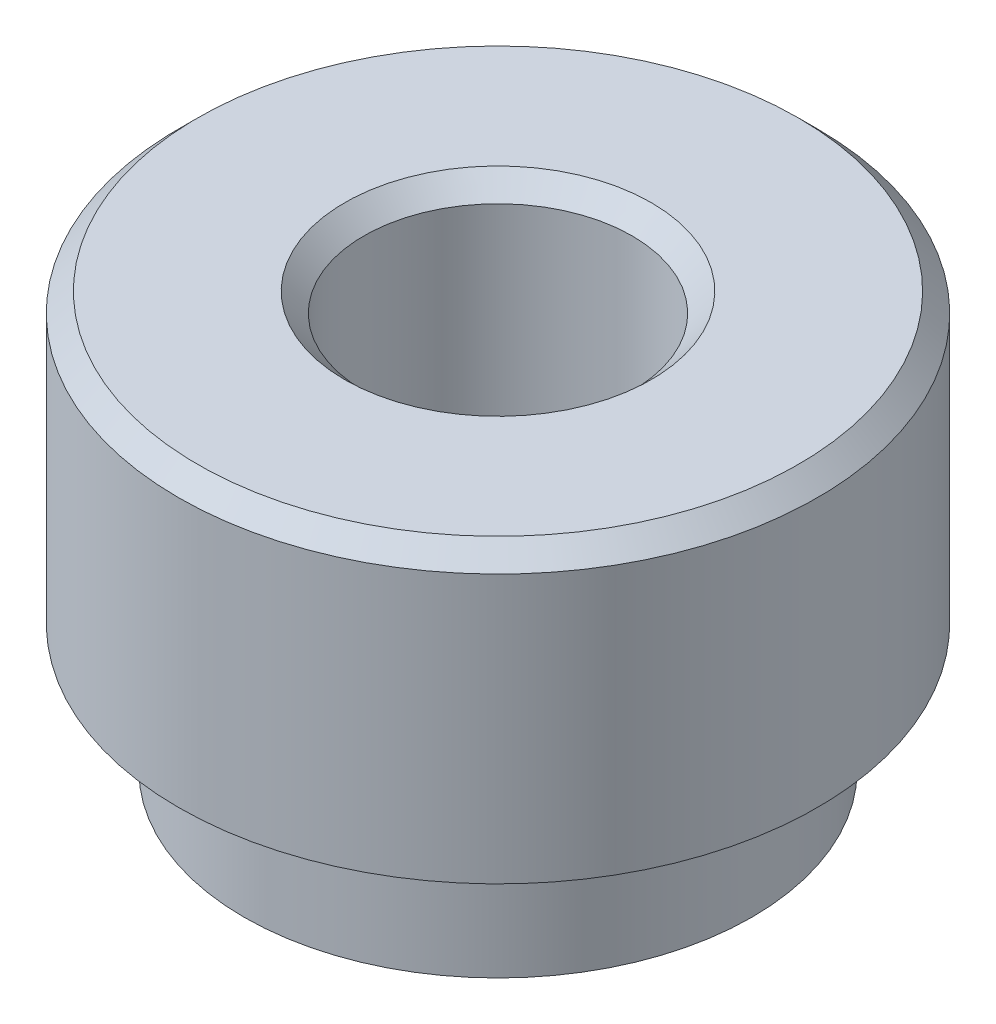
SolidWorks part; units mm, degrees
ref_plane "前视基准面" through (0, 0, 0) normal (0, 0, 1) x (1, 0, 0)
ref_plane "上视基准面" through (0, 0, 0) normal (0, 1, 0) x (1, 0, 0)
ref_plane "右视基准面" through (0, 0, 0) normal (1, 0, 0) x (0, 0, -1)
sketch "草图1" plane through (0, 0, 0) normal (0, 0, 1) x (1, 0, 0)
  line L0 (0, 0) -> (0, 56.263) construction
  line L1 (0, 6.5) -> (-5, 6.5)
  line L2 (-5, 6.5) -> (-5, 2)
  line L3 (-5, 2) -> (-3.975, 2)
  line L4 (-3.975, 2) -> (-3.975, 0)
  line L5 (-3.975, 0) -> (-3.25, 0)
  line L6 (0, 6.5) -> (0, 2)
  line L7 (-3.25, 0) -> (-3.25, 2)
  line L8 (-3.25, 2) -> (0, 2)
  dimension "D1" = 7.95
  dimension "D2" = 10
  dimension "D3" = 2
  dimension "D4" = 6.5
  dimension "D5" = 6.5
revolve "旋转1" add sketch "草图1" angle 360 about L0
hole_wizard "M5 螺纹孔1" positions "草图3" profile "草图4" tap size "M5" standard "GB" end condition through all
sketch "草图3" plane through (0, 6.5, 0) normal (0, 1, 0) x (1, 0, 0)
  point P0 (0, 0)
sketch "草图4" plane through (0, 6.5, 0) normal (1, 0, 0) x (0, 0, 1)
  line L0 (0, 0) -> (0, 6.5)
  line L1 (0, 6.5) -> (2.1, 6.5)
  line L2 (2.1, 6.5) -> (2.1, 0)
  line L5 (2.1, 0) -> (0, 0)
  line L11 (0, -6.35) -> (0, 107.95) construction
  dimension "通孔螺纹孔钻头直径" = 4.2
  dimension "通孔螺纹孔钻头深度" = 6.5
cosmetic thread "孔螺蚊线1" parameters "D2"=5
chamfer "倒角1" distance 0.3 angle 45 3 edges at (0, 6.5, -5) (0, 6.5, 2.1) (0, 2, 2.1)
